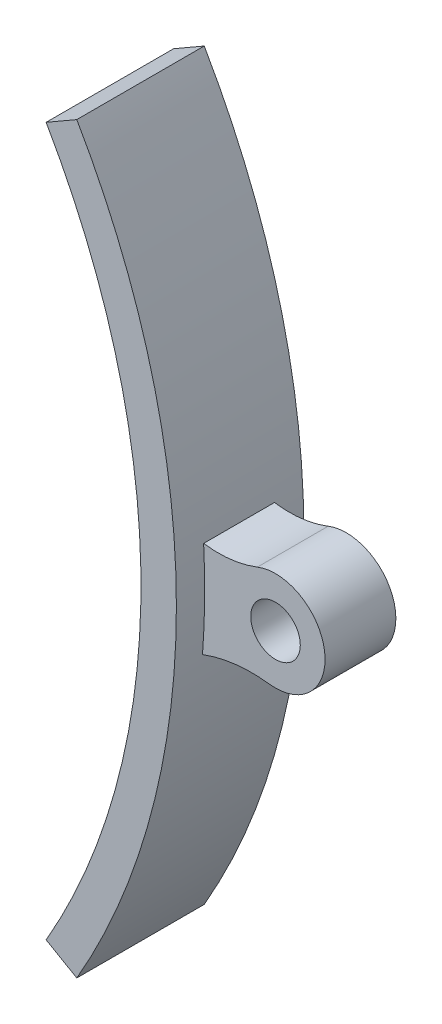
from build123d import *

# Parameters (mm, degrees)
EXTRUDE_1_DEPTH = 18
SKETCH_8_R      = 3.5
EXTRUDE_5_DEPTH = 5


with BuildPart() as part:
    # 草图1 → 凸台-拉伸1 (new body)
    with BuildSketch(Plane.XY):
        with BuildLine():
            Line((86.602540378, 50), (90.932667397, 52.5))
            ThreePointArc((90.932667397, 52.5), (105, 0), (90.932667397, -52.5))
            Line((90.932667397, -52.5), (86.602540378, -50))
            ThreePointArc((86.602540378, -50), (100, 0), (86.602540378, 50))
        make_face()
    extrude(amount=EXTRUDE_1_DEPTH)

    # 草图8 → 凸台-拉伸5 (add, symmetric)
    with BuildSketch(Plane.XY.offset(9)):
        with BuildLine():
            Line((103.468607759, 5.878851187), (102.726389869, -8.907444453))
            ThreePointArc((102.726389869, -8.907444453), (108.287042552, -7.083213633), (114.137686614, -6.946683786))
            ThreePointArc((114.137686614, -6.946683786), (121.944727548, 0.877928973), (112.436089109, 6.513552099))
            ThreePointArc((112.436089109, 6.513552099), (108.00101592, 5.508594665), (103.468607759, 5.878851187))
        make_face()
        with Locations((115, 0)):
            Circle(SKETCH_8_R, mode=Mode.SUBTRACT)
    extrude(amount=EXTRUDE_5_DEPTH, both=True)


solid = part.part
